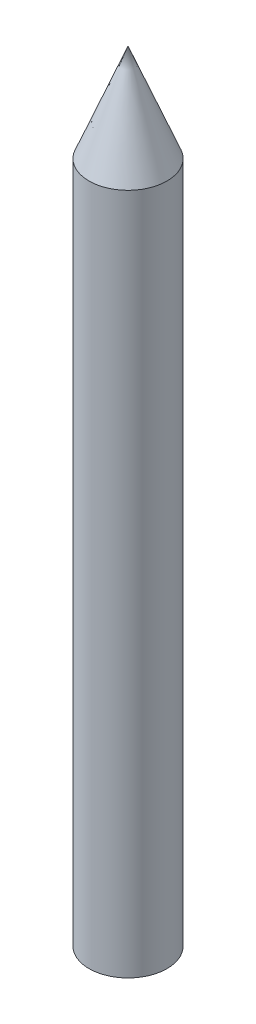
SolidWorks part; units mm, degrees
ref_plane "前视基准面" through (0, 0, 0) normal (0, 0, 1) x (1, 0, 0)
ref_plane "上视基准面" through (0, 0, 0) normal (0, 1, 0) x (1, 0, 0)
ref_plane "右视基准面" through (0, 0, 0) normal (1, 0, 0) x (0, 0, -1)
sketch "草图1" plane through (0, 0, 0) normal (0, 0, 1) x (1, 0, 0)
  line L0 (0, 0) -> (0, 80)
  line L1 (0, 0) -> (-4, 0)
  line L2 (-4, 0) -> (-4, 70)
  line L3 (-4, 70) -> (0, 80)
  dimension "D1" = 4
  dimension "D2" = 80
  dimension "D3" = 70
revolve "旋转1" add sketch "草图1" angle 360 about L0
